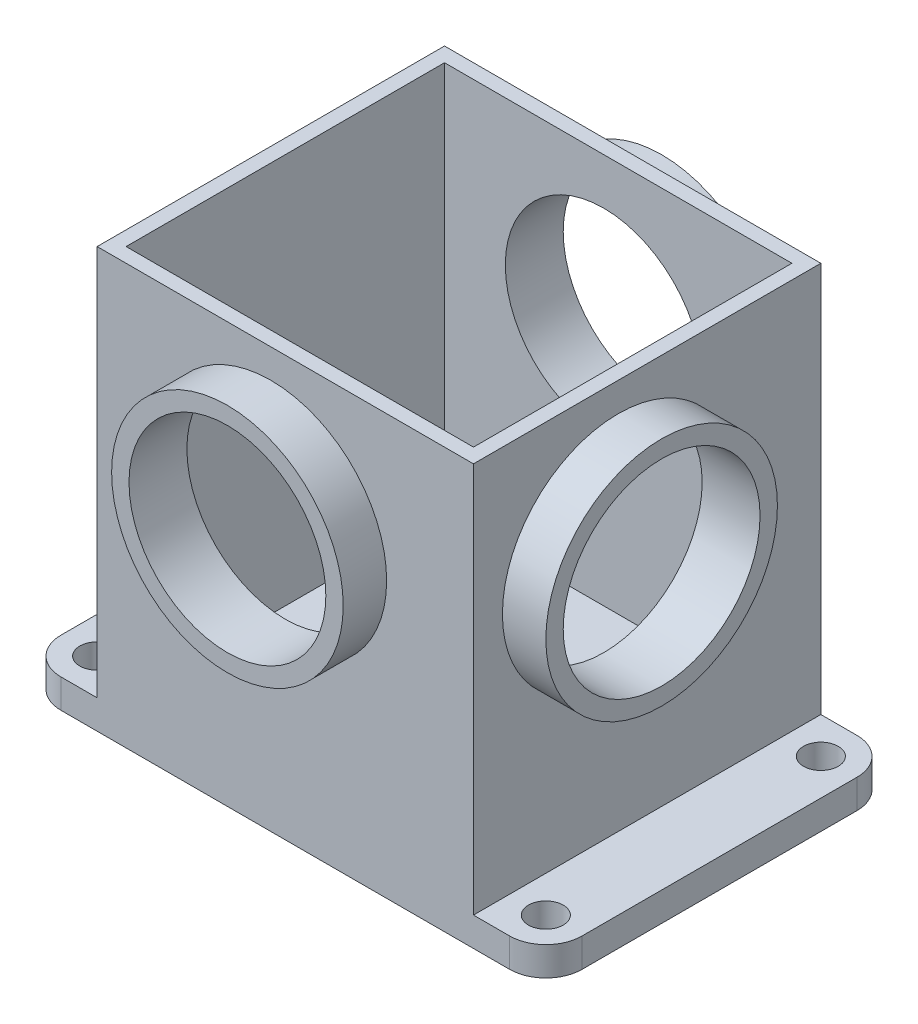
from build123d import *

# Parameters (mm, degrees)
EXTRUDE_1_DEPTH     = 10
SKETCH_2_R          = 6
CUT_EXTRUDE_1_DEPTH = 197.277864264
SKETCH_3_W          = 130
SKETCH_3_H          = 120
SKETCH_3_W_2        = 120
SKETCH_3_H_2        = 110
EXTRUDE_4_DEPTH     = 135
SKETCH_4_R          = 40
EXTRUDE_5_DEPTH     = 15
SKETCH_6_R          = 34
CUT_EXTRUDE_2_DEPTH = 20
SKETCH_7_R          = 40
EXTRUDE_6_DEPTH     = 15
SKETCH_8_R          = 34
CUT_EXTRUDE_3_DEPTH = 20
EXTRUDE_START       = 15
SKETCH_9_R          = 40
EXTRUDE_7_DEPTH     = 15
CUT_EXTRUDE_START   = -20
SKETCH_10_R         = 34
CUT_EXTRUDE_4_DEPTH = 20


with BuildPart() as part:
    # 草图1 → 凸台-拉伸1 (new body)
    with BuildSketch(Plane(origin=(0, 0, 0), x_dir=(1, 0, 0), z_dir=(0, 1, 0))):
        with BuildLine():
            Line((0, 120), (-12.5, 120))
            ThreePointArc((-12.5, 120), (-21.338834765, 116.338834765), (-25, 107.5))
            Line((-25, 107.5), (-25, 12.5))
            ThreePointArc((-25, 12.5), (-21.338834765, 3.661165235), (-12.5, 0))
            Line((-12.5, 0), (0, 0))
            Line((0, 0), (130, 0))
            Line((130, 0), (142.5, 0))
            ThreePointArc((142.5, 0), (151.338834765, 3.661165235), (155, 12.5))
            Line((155, 12.5), (155, 107.5))
            ThreePointArc((155, 107.5), (151.338834765, 116.338834765), (142.5, 120))
            Line((142.5, 120), (130, 120))
            Line((130, 120), (0, 120))
        make_face()
    extrude(amount=EXTRUDE_1_DEPTH)

    # 草图2 → 切除-拉伸1 (cut, through all)
    with BuildSketch(Plane(origin=(0, 10, 0), x_dir=(1, 0, 0), z_dir=(0, 1, 0))):
        with Locations(Location((-12.5, 107.5, 0), (0, 0, 270))):
            Circle(SKETCH_2_R)
        with Locations(Location((142.5, 107.5, 0), (0, 0, 270))):
            Circle(SKETCH_2_R)
        with Locations(Location((142.5, 12.5, 0), (0, 0, 270))):
            Circle(SKETCH_2_R)
        with Locations(Location((-12.5, 12.5, 0), (0, 0, 270))):
            Circle(SKETCH_2_R)
    extrude(amount=-CUT_EXTRUDE_1_DEPTH, mode=Mode.SUBTRACT)

    # 草图3 → 凸台-拉伸4 (add)
    with BuildSketch(Plane(origin=(0, 10, 0), x_dir=(1, 0, 0), z_dir=(0, 1, 0))):
        with Locations((65, 60)):
            Rectangle(SKETCH_3_W, SKETCH_3_H)
        with Locations((65, 60)):
            Rectangle(SKETCH_3_W_2, SKETCH_3_H_2, mode=Mode.SUBTRACT)
    extrude(amount=EXTRUDE_4_DEPTH)

    # 草图4 → 凸台-拉伸5 (add)
    with BuildSketch(Plane.XY):
        with Locations(Location((60, 95, 0), (0, 0, 180))):
            Circle(SKETCH_4_R)
    extrude(amount=EXTRUDE_5_DEPTH)

    # 草图6 → 切除-拉伸2 (cut)
    with BuildSketch(Plane.XY.offset(15)):
        with Locations((60, 95)):
            Circle(SKETCH_6_R)
    extrude(amount=-CUT_EXTRUDE_2_DEPTH, mode=Mode.SUBTRACT)

    # 草图7 → 凸台-拉伸6 (add)
    with BuildSketch(Plane(origin=(130, 0, 0), x_dir=(0, 0, -1), z_dir=(1, 0, 0))):
        with Locations(Location((50, 95, 0), (0, 0, 180))):
            Circle(SKETCH_7_R)
    extrude(amount=EXTRUDE_6_DEPTH)

    # 草图8 → 切除-拉伸3 (cut)
    with BuildSketch(Plane(origin=(145, 0, 0), x_dir=(0, 0, -1), z_dir=(1, 0, 0))):
        with Locations((50, 95)):
            Circle(SKETCH_8_R)
    extrude(amount=-CUT_EXTRUDE_3_DEPTH, mode=Mode.SUBTRACT)

    # 草图9 → 凸台-拉伸7 (add)
    with BuildSketch(Plane(origin=(0, 0, -120), x_dir=(-1, 0, 0), z_dir=(0, 0, -1)).offset(EXTRUDE_START)):
        with Locations((-60, 95)):
            Circle(SKETCH_9_R)
    extrude(amount=-EXTRUDE_7_DEPTH)

    # 草图10 → 切除-拉伸4 (cut)
    with BuildSketch(Plane(origin=(0, 0, -135), x_dir=(-1, 0, 0), z_dir=(0, 0, -1)).offset(CUT_EXTRUDE_START)):
        with Locations(Location((-60, 95, 0), (0, 0, 180))):
            Circle(SKETCH_10_R)
    extrude(amount=CUT_EXTRUDE_4_DEPTH, mode=Mode.SUBTRACT)


solid = part.part
